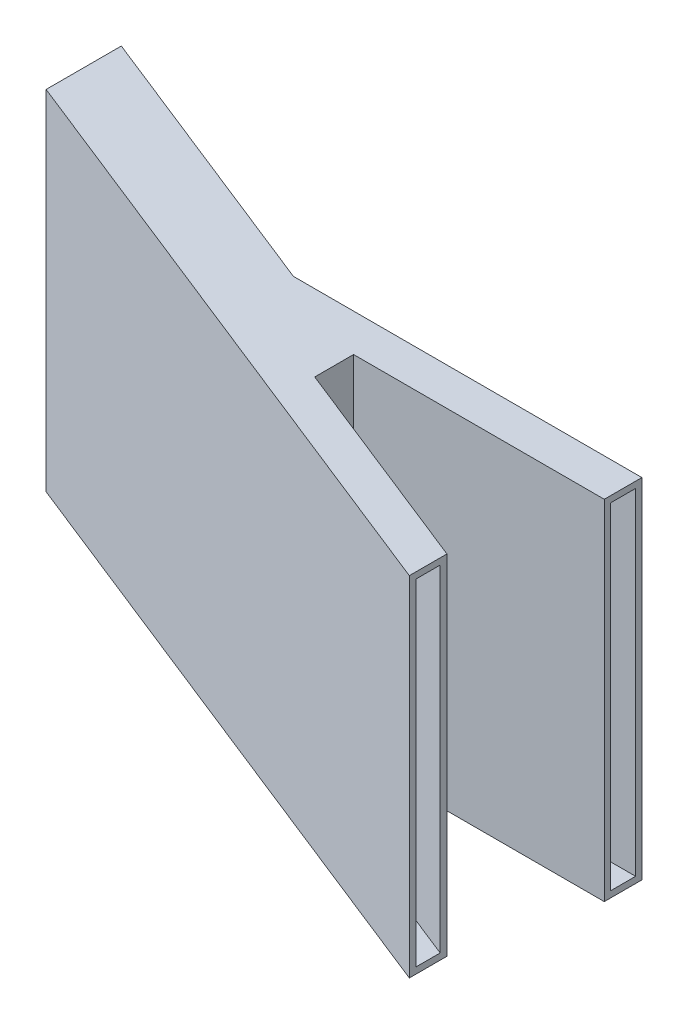
SolidWorks part; units mm, degrees
ref_plane "Front" through (0, 0, 0) normal (0, 0, 1) x (1, 0, 0)
ref_plane "Top" through (0, 0, 0) normal (0, 1, 0) x (1, 0, 0)
ref_plane "Right" through (0, 0, 0) normal (1, 0, 0) x (0, 0, -1)
sketch "Sketch1" plane through (0, 0, 0) normal (0, 1, 0) x (1, 0, 0)
  line L0 (100, 0) -> (500, 0)
  line L1 (500, 0) -> (500, 60)
  line L2 (500, 60) -> (-56, 60)
  line L3 (-56, 60) -> (-511.5932, 241.0169)
  line L4 (-511.5932, 241.0169) -> (-511.5932, 121.0169)
  line L5 (-511.5932, 121.0169) -> (450, -261.0446)
  line L6 (450, -261.0446) -> (450, -201.0446)
  line L7 (450, -201.0446) -> (100, -61.9821)
  line L8 (100, 0) -> (100, -61.9821)
  dimension "D1" = 60
  dimension "D2" = 556
  dimension "D3" = 50
  dimension "D4" = 0
  dimension "D5" = 120
  dimension "D6" = 60
  dimension "D7" = 400
  dimension "D8" = 0
extrude "Boss-Extrude1" add sketch "Sketch1" along normal blind 556
shell "Shell1" thickness 10
sketch "Sketch2" plane through (0, 0, -60) normal (0, 0, -1) x (-1, 0, 0)
  line L0 (56, 556) -> (56, 0) construction
  line L1 (56, 41.0956) -> (-44, 41.0956)
  line L2 (56, 41.0956) -> (56, 485.3323)
  line L3 (56, 485.3323) -> (-44, 485.3323)
  line L4 (-44, 41.0956) -> (-44, 485.3323)
  dimension "D1" = 100
extrude "Cut-Extrude1" cut sketch "Sketch2" against normal blind 15
